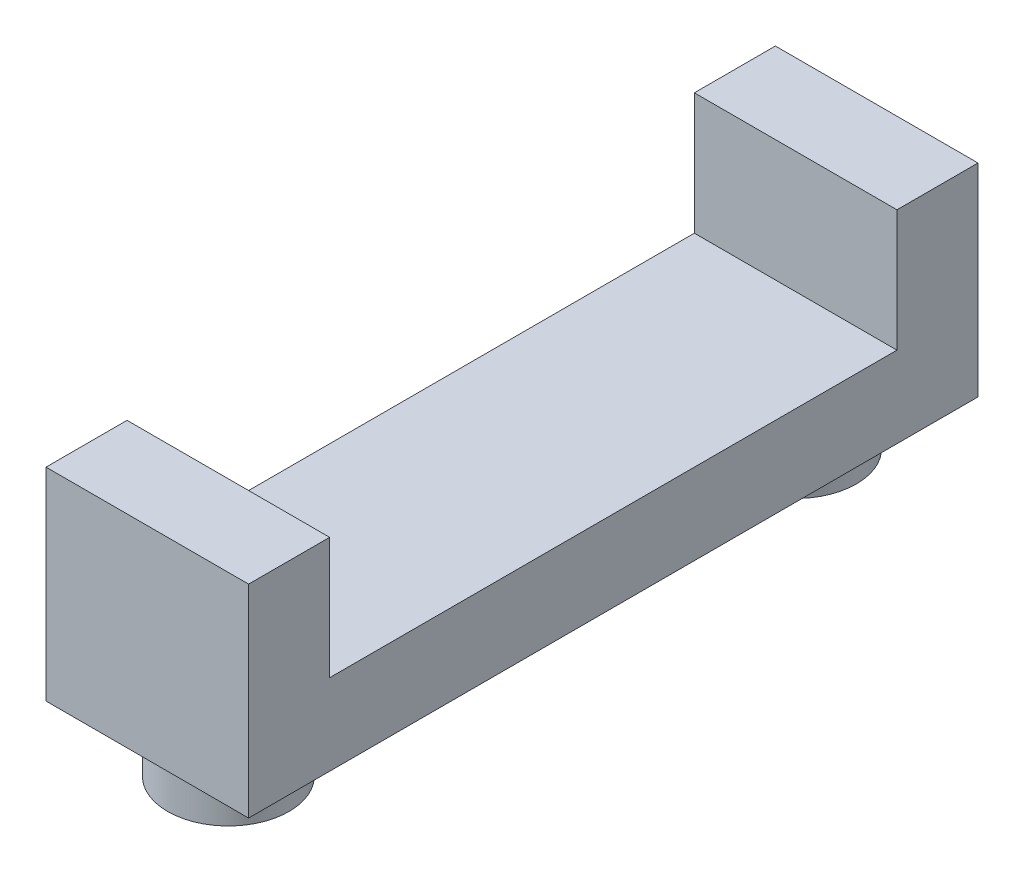
from build123d import *

# Parameters (mm, degrees)
SKETCH1_W           = 500
SKETCH1_H           = 500
BOSS_EXTRUDE1_DEPTH = 900
SKETCH2_R           = 150
BOSS_EXTRUDE2_DEPTH = 136
SKETCH3_W           = 1400
SKETCH3_H           = 300
CUT_EXTRUDE1_DEPTH  = 1100.543541657


with BuildPart() as part:
    # Sketch1 → Boss-Extrude1 (new, symmetric)
    with BuildSketch(Plane.XY):
        Rectangle(SKETCH1_W, SKETCH1_H)
    extrude(amount=BOSS_EXTRUDE1_DEPTH, both=True)

    # Sketch2 → Boss-Extrude2 (add)
    with BuildSketch(Plane.XZ.offset(250)):
        with Locations(Location((0, -700, 0), (0, 0, 90))):
            Circle(SKETCH2_R)
        with Locations(Location((0, 700, 0), (0, 0, 90))):
            Circle(SKETCH2_R)
    extrude(amount=BOSS_EXTRUDE2_DEPTH)

    # Sketch3 → Cut-Extrude1 (cut, through all)
    with BuildSketch(Plane(origin=(250, 0, 0), x_dir=(0, 0, -1), z_dir=(1, 0, 0))):
        with Locations((0, 100)):
            Rectangle(SKETCH3_W, SKETCH3_H)
    extrude(amount=-CUT_EXTRUDE1_DEPTH, mode=Mode.SUBTRACT)


solid = part.part
